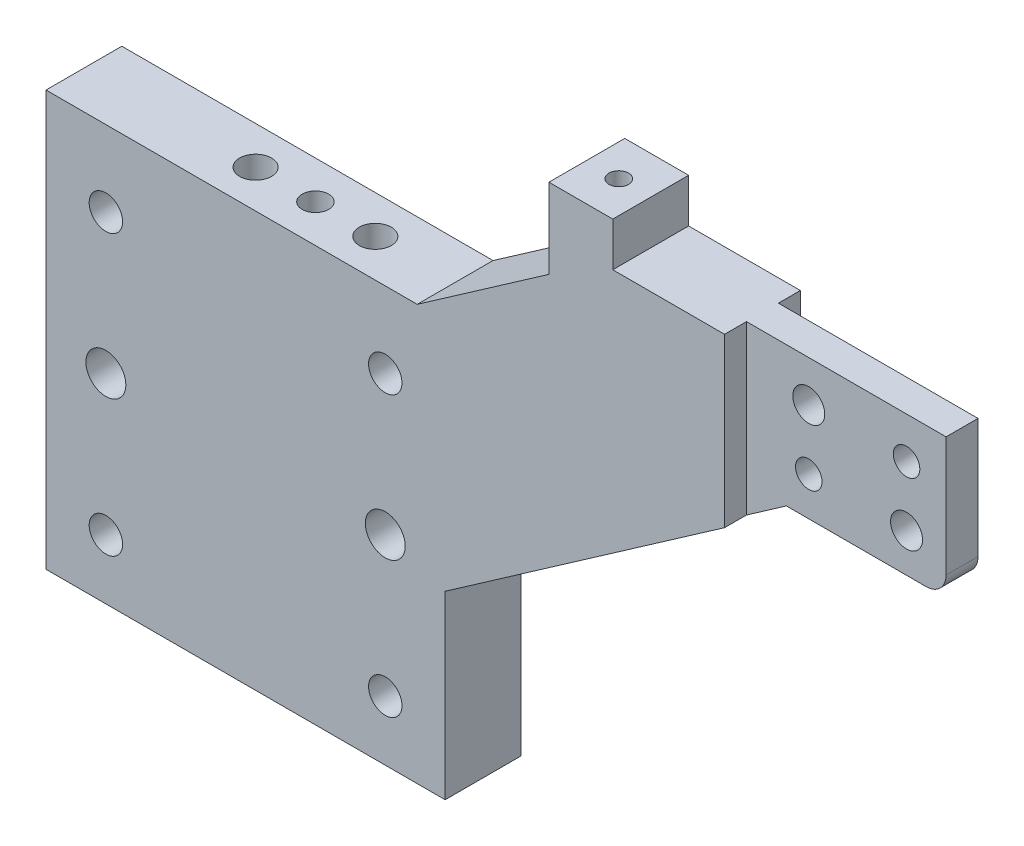
from build123d import *

# Parameters (mm, degrees)
SKETCH1_R           = 4.188
SKETCH1_R_2         = 5
SKETCH1_R_3         = 3.3235
SKETCH1_R_4         = 4
BOSS_EXTRUDE1_DEPTH = 19
SKETCH2_R           = 4
SKETCH2_R_2         = 3.325
CUT_EXTRUDE1_DEPTH  = 15
SKETCH3_R           = 2.4585
CUT_EXTRUDE2_DEPTH  = 15
SKETCH4_W           = 50
SKETCH4_H           = 41.969696972
CUT_EXTRUDE3_DEPTH  = 5.5
SKETCH5_W           = 50
SKETCH5_H           = 41.969696972
CUT_EXTRUDE4_DEPTH  = 5.5
FILLET1_R           = 5


with BuildPart() as part:
    # Sketch1 → Boss-Extrude1 (new body)
    with BuildSketch(Plane.XY):
        Polygon((0, 0), (0, 104.0002829), (93, 104.0002829), (126, 127.0002829), (126, 147.0002829), (142, 147.0002829), (142, 136.0002829), (220, 136.0002829), (220, 101.000282896), (179.999999997, 101.000282896), (100, 45.24270714), (100, 0), align=None)
        with Locations((15, 15)):
            Circle(SKETCH1_R, mode=Mode.SUBTRACT)
        with Locations((15, 50)):
            Circle(SKETCH1_R_2, mode=Mode.SUBTRACT)
        with Locations((15, 85)):
            Circle(SKETCH1_R, mode=Mode.SUBTRACT)
        with Locations((85, 85)):
            Circle(SKETCH1_R, mode=Mode.SUBTRACT)
        with Locations((85, 50)):
            Circle(SKETCH1_R_2, mode=Mode.SUBTRACT)
        with Locations((85, 15)):
            Circle(SKETCH1_R, mode=Mode.SUBTRACT)
        with Locations((210.1, 125.7002829)):
            Circle(SKETCH1_R_3, mode=Mode.SUBTRACT)
        with Locations((210.1, 110.7002829)):
            Circle(SKETCH1_R_4, mode=Mode.SUBTRACT)
        with Locations((185.6, 110.7002829)):
            Circle(SKETCH1_R_3, mode=Mode.SUBTRACT)
        with Locations((185.6, 125.7002829)):
            Circle(SKETCH1_R_4, mode=Mode.SUBTRACT)
    extrude(amount=BOSS_EXTRUDE1_DEPTH)

    # Sketch2 → Cut-Extrude1 (cut)
    with BuildSketch(Plane(origin=(0, 104.0002829, 0), x_dir=(1, 0, 0), z_dir=(0, 1, 0))):
        with Locations(Location((43, -9.5, 0), (0, 0, 270))):
            Circle(SKETCH2_R)
        with Locations(Location((58, -9.5, 0), (0, 0, 270))):
            Circle(SKETCH2_R_2)
        with Locations(Location((73, -9.5, 0), (0, 0, 270))):
            Circle(SKETCH2_R)
    extrude(amount=-CUT_EXTRUDE1_DEPTH, mode=Mode.SUBTRACT)

    # Sketch3 → Cut-Extrude2 (cut)
    with BuildSketch(Plane(origin=(0, 147.0002829, 0), x_dir=(1, 0, 0), z_dir=(0, 1, 0))):
        with Locations(Location((134, -9.5, 0), (0, 0, 270))):
            Circle(SKETCH3_R)
    extrude(amount=-CUT_EXTRUDE2_DEPTH, mode=Mode.SUBTRACT)

    # Sketch4 → Cut-Extrude3 (cut)
    with BuildSketch(Plane.XY.offset(19)):
        with Locations((195, 115.015434414)):
            Rectangle(SKETCH4_W, SKETCH4_H)
    extrude(amount=-CUT_EXTRUDE3_DEPTH, mode=Mode.SUBTRACT)

    # Sketch5 → Cut-Extrude4 (cut)
    with BuildSketch(Plane(origin=(0, 0, 0), x_dir=(-1, 0, 0), z_dir=(0, 0, -1))):
        with Locations((-195, 115.015434414)):
            Rectangle(SKETCH5_W, SKETCH5_H)
    extrude(amount=-CUT_EXTRUDE4_DEPTH, mode=Mode.SUBTRACT)

    # Fillet1
    fillet1_edges = [part.edges().sort_by_distance(p)[0] for p in [
        (220, 101.000282896, 9.5),
    ]]
    fillet(fillet1_edges, radius=FILLET1_R)


solid = part.part
